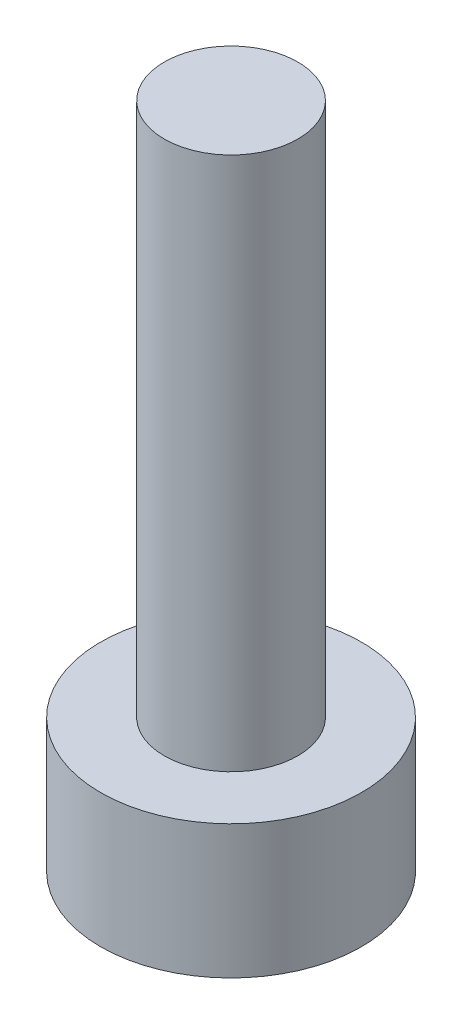
from build123d import *

# Parameters (mm, degrees)
SKETCH2_R           = 2.93
BOSS_EXTRUDE1_DEPTH = 3
SKETCH3_R           = 1.5
BOSS_EXTRUDE2_DEPTH = 12
CUT_EXTRUDE1_DEPTH  = 1.3


with BuildPart() as part:
    # Sketch2 → Boss-Extrude1 (new body)
    with BuildSketch(Plane(origin=(0, 0, 0), x_dir=(1, 0, 0), z_dir=(0, 1, 0))):
        with Locations(Location((0, 0, 0), (0, 0, 270))):
            Circle(SKETCH2_R)
    extrude(amount=BOSS_EXTRUDE1_DEPTH)

    # Sketch3 → Boss-Extrude2 (add)
    with BuildSketch(Plane(origin=(0, 3, 0), x_dir=(1, 0, 0), z_dir=(0, 1, 0))):
        with Locations(Location((0, 0, 0), (0, 0, 270))):
            Circle(SKETCH3_R)
    extrude(amount=BOSS_EXTRUDE2_DEPTH)

    # Sketch4 → Cut-Extrude1 (cut)
    with BuildSketch(Plane.XZ):
        Polygon((0.989792051, 0.827291784), (-0.221559676, 1.270830953), (-1.211351727, 0.443539168), (-0.989792051, -0.827291784), (0.221559676, -1.270830953), (1.211351727, -0.443539168), align=None)
    extrude(amount=-CUT_EXTRUDE1_DEPTH, mode=Mode.SUBTRACT)


solid = part.part
